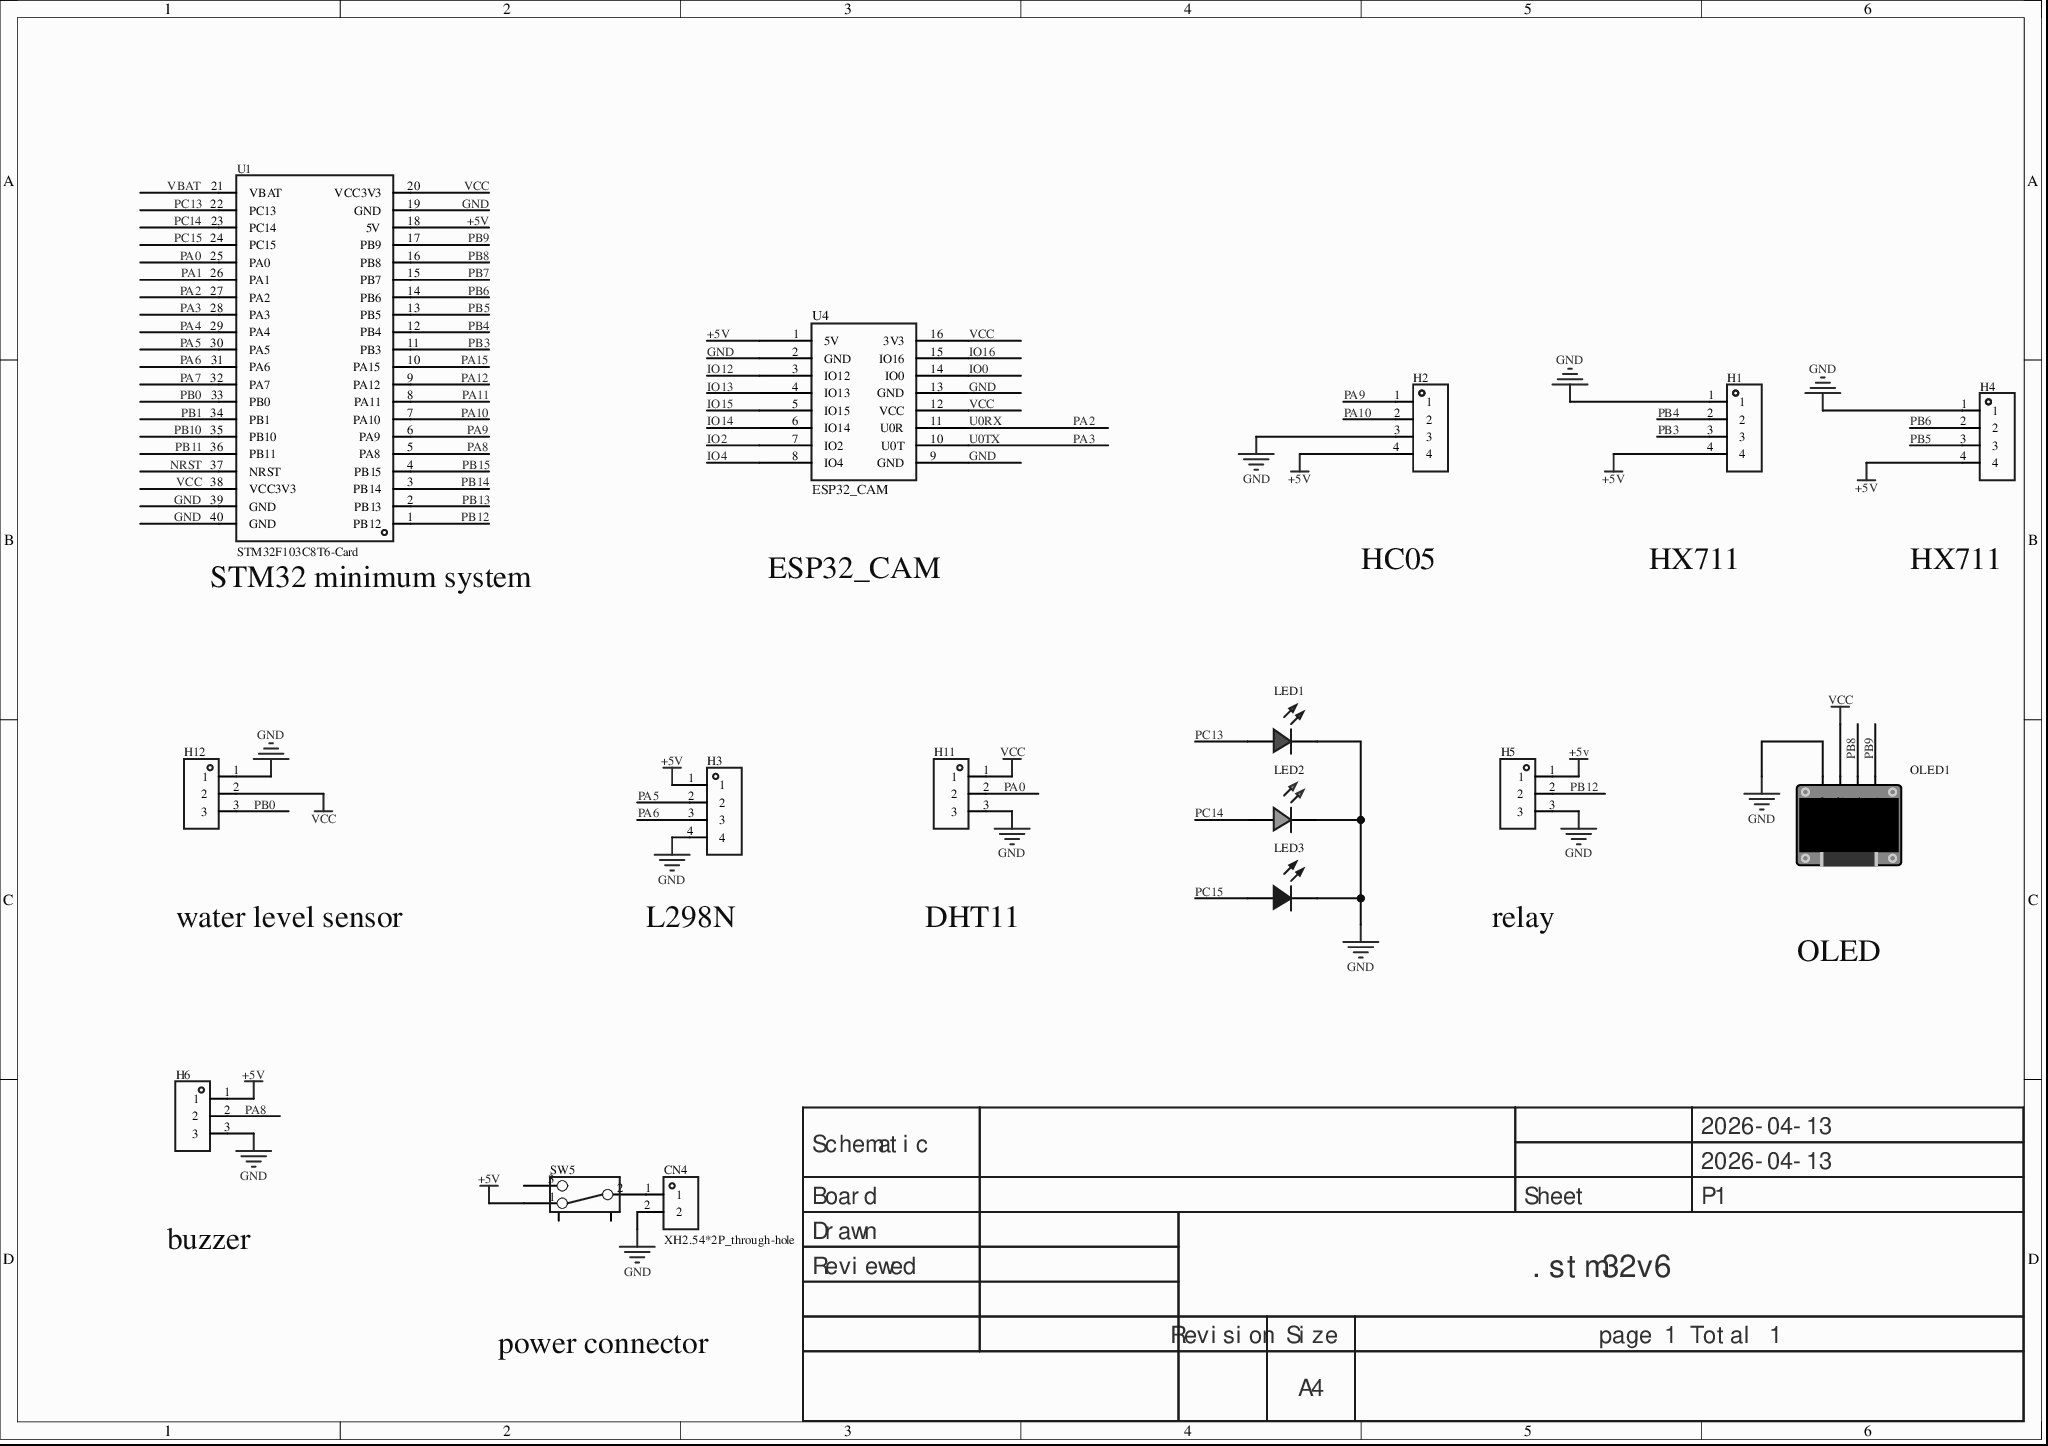
[diagram p0: MISC52091-3.schdoc]
# Altium project MISC52091-2.PrjPcb
1 sheet, 16 parts. Net scope: global (net labels, ports and power ports of the same name join across sheets).
Board file: MISC52091.pcbdoc

## Sheet MISC52091-3.schdoc
size 297 x 209 mm; Version: V1.0; @Project Name: MISC52091; @Page Count: 1; @Update Date: 2026-04-13; @Create Date: 2026-04-13; @Schematic Name: MISC52091; @Page No: 1; @Create Time: 23:22:16; @Update Time: 17:32:40; @Board Name: MISC52091

### Parts
CN4  XH2.54*2P_through-hole  [CONN-TH_2P-P2.50-XH2.54-2P]
H1  (no value)  [HDR-TH_4P-P2.54-V-F]
H2  (no value)  [HDR-TH_4P-P2.54-V-F]
H3  (no value)  [HDR-TH_4P-P2.54-V-M]
H4  (no value)  [HDR-TH_4P-P2.54-V-F]
H5  (no value)  [HDR-TH_3P-P2.54-V-F]
H6  (no value)  [HDR-TH_3P-P2.54-V-F]
H11  (no value)  [HDR-TH_3P-P2.54-V-F]
H12  (no value)  [HDR-TH_3P-P2.54-V-F]
LED1  (no value)  [LED_TH-3mm]
LED2  (no value)  [LED_TH-3mm]
LED3  (no value)  [LED_TH-3mm]
OLED1  (no value)  [0.96OLED_4P]
SW5  (no value)  [拨动开关]
U1  STM32F103C8T6-Card  [CONN-TH_L53.3-W22.9_STM32F103C8T6-CARD]
U4  ESP32_CAM  [ESP32-CAM]

### Nets
+5V: H1.4 H2.4 H3.1 H4.4 H5.1 H6.1 SW5.1 U1.18(5V) U4.1(5V)
GND: CN4.2 H1.1 H2.3 H3.4 H4.1 H5.3 H6.3 H11.3 H12.1 LED1.2(A) LED2.2(A) LED3.2(A) OLED1.1(GND) U1.19(GND) U1.39(GND) U1.40(GND) U4.2(GND) U4.9(GND) U4.13(GND)
VCC: H11.1 H12.2 OLED1.2(VCC) U1.20(VCC3V3) U1.38(VCC3V3) U4.12(VCC) U4.16(3V3)
IO0: U4.14(IO0)
IO2: U4.7(IO2)
IO4: U4.8(IO4)
IO12: U4.3(IO12)
IO13: U4.4(IO13)
IO14: U4.6(IO14)
IO15: U4.5(IO15)
IO16: U4.15(IO16)
NRST: U1.37(NRST)
PA0: H11.2 U1.25(PA0)
PA1: U1.26(PA1)
PA2: U1.27(PA2) U4.11(U0R)  [also labelled U0RX]
PA3: U1.28(PA3) U4.10(U0T)  [also labelled U0TX]
PA4: U1.29(PA4)
PA5: H3.2 U1.30(PA5)
PA6: H3.3 U1.31(PA6)
PA7: U1.32(PA7)
PA8: H6.2 U1.5(PA8)
PA9: H2.1 U1.6(PA9)
PA10: H2.2 U1.7(PA10)
PA11: U1.8(PA11)
PA12: U1.9(PA12)
PA15: U1.10(PA15)
PB0: H12.3 U1.33(PB0)
PB1: U1.34(PB1)
PB3: H1.3 U1.11(PB3)
PB4: H1.2 U1.12(PB4)
PB5: H4.3 U1.13(PB5)
PB6: H4.2 U1.14(PB6)
PB7: U1.15(PB7)
PB8: OLED1.3(SCL) U1.16(PB8)
PB9: OLED1.4(SDA) U1.17(PB9)
PB10: U1.35(PB10)
PB11: U1.36(PB11)
PB12: H5.2 U1.1(PB12)
PB13: U1.2(PB13)
PB14: U1.3(PB14)
PB15: U1.4(PB15)
PC13: LED1.1(C) U1.22(PC13)
PC14: LED2.1(C) U1.23(PC14)
PC15: LED3.1(C) U1.24(PC15)
VBAT: U1.21(VBAT)
NetCN4_1: CN4.1 SW5.2

Not connected (* = marked no-connect by the designer): SW5 3 4 5

### Notes on the sheet
- (near U1) STM32 minimum system
- ESP32_CAM
- HC05
- HX711
- water level sensor
- (near H3) L298N
- DHT11
- relay
- OLED
- buzzer
- power connector
- Labels drawn without touching a wire or pin: VCC
- 2026-04-13
- Schematic
- Board
- Sheet
- P1
- Drawn
- Reviewed
- .stm32v6
- Revision
- Size
- A4
- page 1 Total 1

### Library data of the parts
CN4 = XH2.54*2P_直插: 3D Model: 325c595e30db4df8abe76612dd40b0fa0819f05c4eef4c71ace90d822a990e87; 3D Model Transform: 295.275,228.346,0,180,0,0,-0.002,-20.079,-137.795; AddInBom: yes; Symbol: XH2.54*2P_through-hole; Device: XH2.54*2P_through-hole; LCSC Part Name: XH2.54*2P_直插; Supplier Part: C9900008615; Manufacturer Part: XH2.54*2P_直插; Supplier Footprint: XH2.54_2P; JLCPCB Part Class: Extended Part; Supplier: LCSC; ConvertToPcb: yes; FootprintName: CONN-TH_2P-P2.50-XH2.54-2P; ModelName: CONN-TH_2P-P2.50-XH2.54-2P
H1 H2 H4 = HDR-F_2.54_1x4P: Symbol: 2.54-1*4P female; 3D Model: d187812051054f85879fcaa51a310d8e0819f05c4eef4c71ace90d822a990e87; 3D Model Transform: 419.6842,98.464,0,0,0,0,0,0,-118.11; ConvertToPcb: yes; Device: HDR-F_2.54_1x4P; Supplier Part: C2718488; Supplier Footprint: 插件; FootprintName: HDR-TH_4P-P2.54-V-F; AddInBom: yes; ModelName: HDR-TH_4P-P2.54-V-F
H3 = HDR-M_2.54_1x4P: Symbol: PZ254V-11-04P; ConvertToPcb: yes; ModelId: 112f4d05e8d64e99ab9a333894bea4f90819f05c4eef4c71ace90d822a990e87; ModelName: HDR-TH_4P-P2.54-M-LI-1X4P; ModelTransform: 399.999,104.7242,0,0,0,0,0,0,-118.11; Device: HDR-M_2.54_1x4P; AddInBom: yes; SupplierPart: C492403; Supplier Footprint: 插件; FootprintName: HDR-TH_4P-P2.54-V-M
H5 H6 H11 H12 = HDR-F_2.54_1x3P: Symbol: PM254V-11-03-H85; 3D Model: f3b3cc5aae9641bf9e56fc160cef875b; 3D Model Transform: 299.9994,100,0,0,0,0,0,0,-118.11; ConvertToPcb: yes; ModelName: HDR2.54-F-LI-1X3P; Device: HDR-F_2.54_1x3P; Supplier Part: C541850; Supplier Footprint: 插件; AddInBom: yes; FootprintName: HDR-TH_3P-P2.54-V-F
LED1 = LED_TH-R_3mm: ConvertToPcb: yes; ModelId: a497c992633541038a38947cdc58012f0819f05c4eef4c71ace90d822a990e87; ModelName: LED-TH-3mm_R; ModelTransform: 141.274,153.327,0,0,0,0,-5.984,0,-137.795; Symbol: LED_TH-R; Device: LED_TH-R_3mm; AddInBom: yes; FootprintName: LED_TH-3mm; Supplier Footprint: 插件
LED2 = LED_TH-G_3mm: AddInBom: yes; ModelId: 07c881668c9448ef9b36eb6a2126ca130819f05c4eef4c71ace90d822a990e87; ModelName: LED-TH-3mm_G; ModelTransform: 141.27444,153.32669525336098,354.32999763315956,0,0,0,-5.90551,0,-137.79528; Symbol: LED_TH-G; Device: LED_TH-G_3mm; ConvertToPcb: yes; FootprintName: LED_TH-3mm; Supplier Footprint: 插件
LED3 = LED_TH-B_3mm: ConvertToPcb: yes; ModelId: ff771fff7070432ca3f353cf0f67af4c0819f05c4eef4c71ace90d822a990e87; ModelName: LED-TH_BD3.8-P2.54-FD_BLUE; ModelTransform: 134.36,149.37,405.47,0,0,0,-11.81,0,-196.85; Symbol: LED_TH-B; Device: LED_TH-B_3mm; AddInBom: yes; Supplier Footprint: 插件; FootprintName: LED_TH-3mm
OLED1 = 0.96OLED模块_4P: Symbol: 0.96OLED module_4P; ConvertToPcb: yes; ModelId: 79c000fdb68d45a296c2e9bedf4f9055; ModelTransform: 1393.69792,1318.895,0,0,0,0,0,-560.079,-137.795; Device: 0.96OLED module_4P; AddInBom: yes; FootprintName: 0.96OLED_4P; Supplier Footprint: 插件; ModelName: 0.96OLED_4P
SW5 = 拨动开关_正: Symbol: toggle switch; Device: toggle switch_positive; ConvertToPcb: yes; ModelId: 4321fe59a4074cbfb4989553f297c68f0819f05c4eef4c71ace90d822a990e87; ModelName: SW-TH_SS-12D02-VG4; ModelTransform: 370.09,208.7,472.35,0,0,0,0,0,-110; AddInBom: yes; Supplier Footprint: 插件; FootprintName: toggle switch
U1 = STM32F103C8T6-Card: AddInBom: yes; Symbol: STM32F103C8T6-CARD; Device: STM32F103C8T6-Card; LCSC Part Name: STM32F103C8T6-Card; SupplierPart: C9900077949; ManufacturerPart: STM32F103C8T6-Card; Supplier Footprint: 插件; Supplier: LCSC; ConvertToPcb: yes; FootprintName: CONN-TH_L53.3-W22.9_STM32F103C8T6-CARD
U4 = ESP32_CAM: ESP32-CAM module; AddInBom: yes; Symbol: ESP32_CAM; Device: ESP32_CAM; Origin Footprint: ESP32-CAM; FootprintName: ESP32-CAM; ConvertToPcb: yes